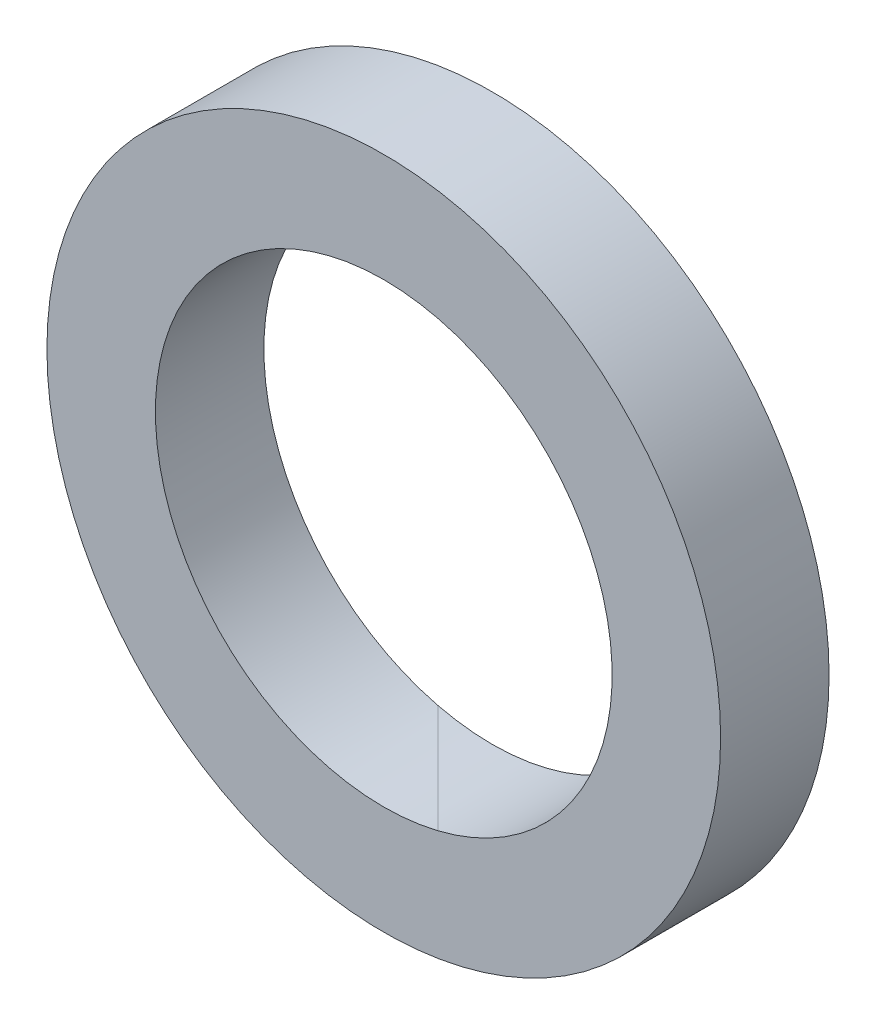
SolidWorks part; units mm, degrees
ref_plane "Front Plane" through (0, 0, 0) normal (0, 0, 1) x (1, 0, 0)
ref_plane "Top Plane" through (0, 0, 0) normal (0, 1, 0) x (1, 0, 0)
ref_plane "Right Plane" through (0, 0, 0) normal (1, 0, 0) x (0, 0, -1)
sketch "Sketch1" plane through (0, 0, 0) normal (0, 0, 1) x (1, 0, 0)
  circle A0 centre (0, 0) radius 20
  circle A1 centre (0, 0) radius 29.5
  dimension "D1" = 40
  dimension "D2" = 9.5
extrude "Boss-Extrude1" add sketch "Sketch1" along normal blind 9.5
sketch "Sketch2" plane through (0, 0, 0) normal (0, 1, 0) x (1, 0, 0)
  line L0 (-4.75, 0) -> (4.75, -9.5)
  line L1 (-32.45, 0) -> (32.45, 0) construction
  line L2 (0, -5.225) -> (0, 5.225) construction
  line L3 (-29.5, -9.5) -> (29.5, -9.5) construction
  line L4 (0, 0) -> (0, -4.75) construction
  dimension "D1" = 45
split line "Split Line1"
